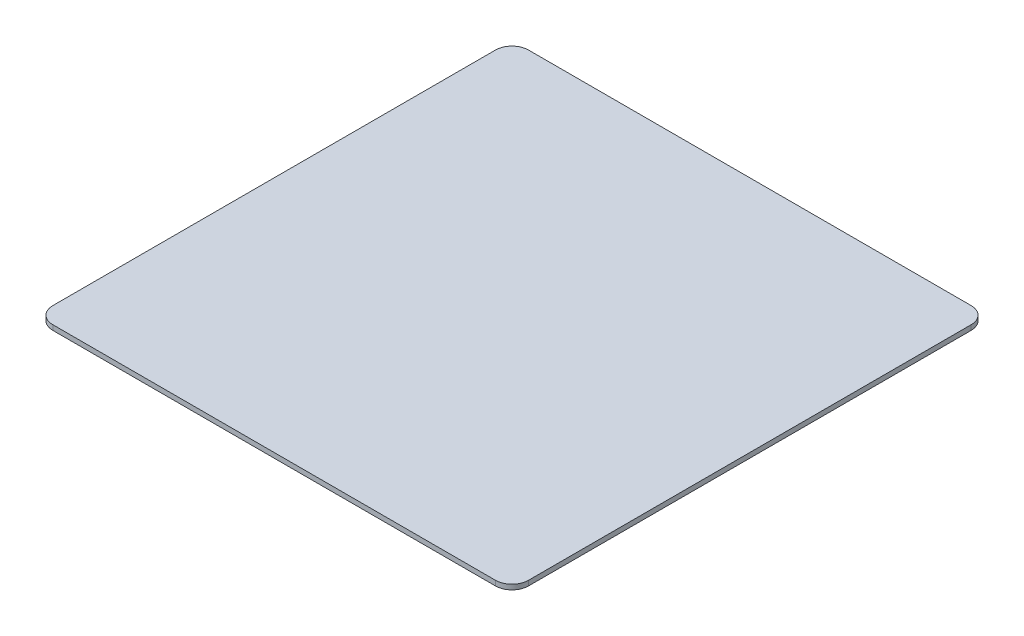
SolidWorks part; units mm, degrees
ref_plane "Front Plane" through (0, 0, 0) normal (0, 0, 1) x (1, 0, 0)
ref_plane "Top Plane" through (0, 0, 0) normal (0, 1, 0) x (1, 0, 0)
ref_plane "Right Plane" through (0, 0, 0) normal (1, 0, 0) x (0, 0, -1)
sketch "Sketch1" plane through (0, 0, 0) normal (0, 1, 0) x (1, 0, 0)
  line L1 (-134, -144) -> (134, -144)
  line L2 (-144, -134) -> (-144, 134)
  line L3 (-134, 144) -> (134, 144)
  line L4 (144, -134) -> (144, 134)
  line L5 (-144, -144) -> (144, 144) construction
  line L6 (-144, 144) -> (144, -144) construction
  arc A0 (-134, -144) -> (-144, -134) centre (-134, -134) cw
  arc A1 (134, -144) -> (144, -134) centre (134, -134) ccw
  arc A2 (134, 144) -> (144, 134) centre (134, 134) cw
  arc A3 (-144, 134) -> (-134, 144) centre (-134, 134) cw
  point P0 (0, 0)
  dimension "D3" = 10
  dimension "D1" = 288
  dimension "D2" = 288
extrude "Boss-Extrude1" add sketch "Sketch1" along normal blind 3
